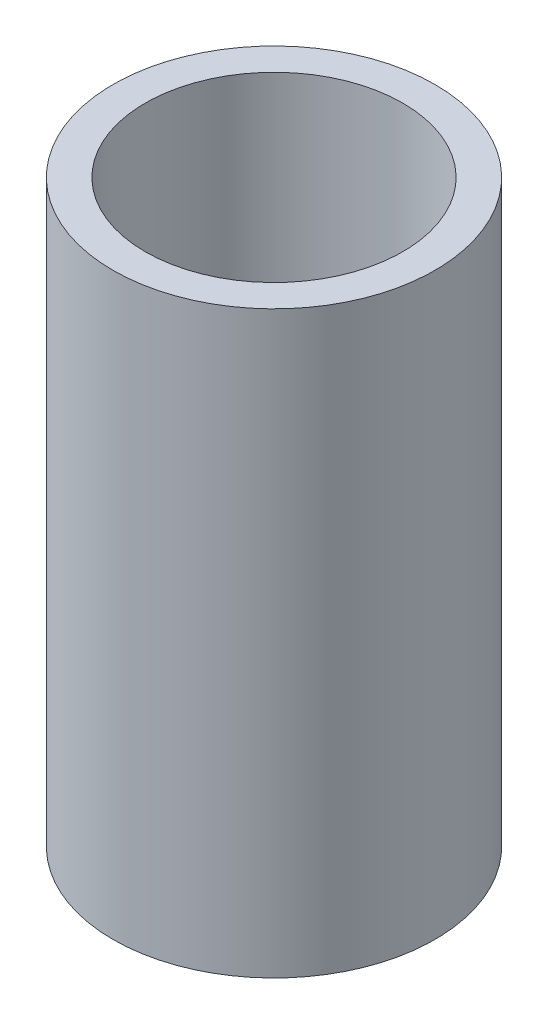
from build123d import *

# Parameters (mm, degrees)
SKETCH1_R           = 10
SKETCH1_R_2         = 8
BOSS_EXTRUDE1_DEPTH = 36


with BuildPart() as part:
    # Sketch1 → Boss-Extrude1 (new body)
    with BuildSketch(Plane(origin=(0, 0, 0), x_dir=(1, 0, 0), z_dir=(0, 1, 0))):
        with Locations(Location((0, 0, 0), (0, 0, 270))):
            Circle(SKETCH1_R)
        with Locations(Location((0, 0, 0), (0, 0, 270))):
            Circle(SKETCH1_R_2, mode=Mode.SUBTRACT)
    extrude(amount=BOSS_EXTRUDE1_DEPTH)


solid = part.part
